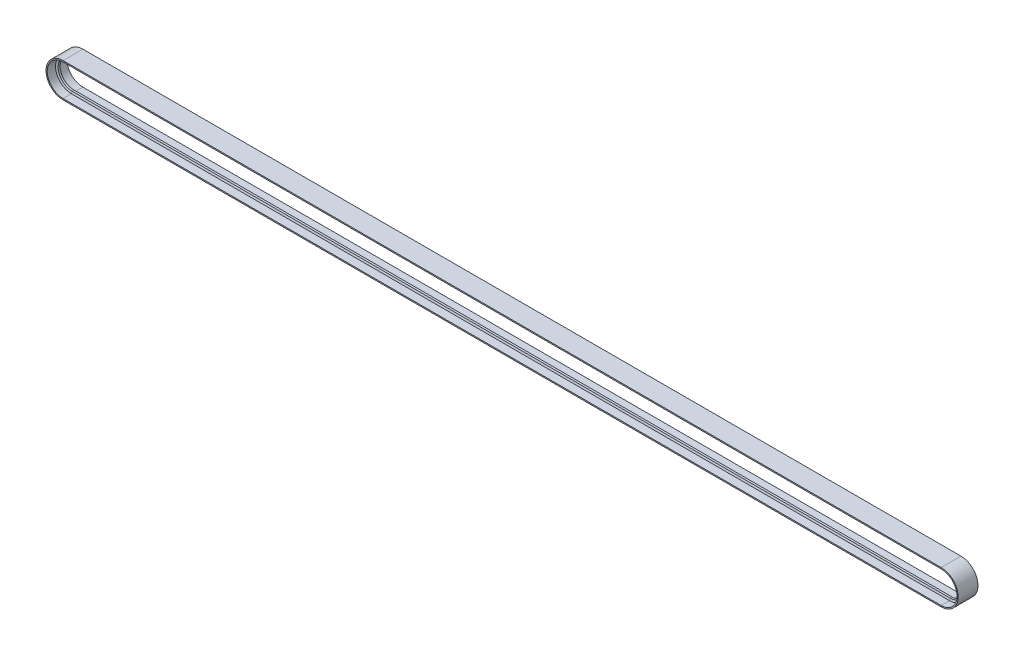
SolidWorks part; units mm, degrees
ref_plane "前视基准面" through (0, 0, 0) normal (0, 0, 1) x (1, 0, 0)
ref_plane "上视基准面" through (0, 0, 0) normal (0, 1, 0) x (1, 0, 0)
ref_plane "右视基准面" through (0, 0, 0) normal (1, 0, 0) x (0, 0, -1)
sketch "草图1" plane through (0, 0, 0) normal (0, 0, 1) x (1, 0, 0)
  line L0 (1108.5, 0) -> (-1108.5, 0) construction
  line L1 (0, 0) -> (0, 99.369) construction
  line L2 (-1108.5, 43) -> (1108.5, 43)
  line L3 (-1108.5, -43) -> (1108.5, -43)
  arc A0 (-1108.5, 43) -> (-1108.5, -43) centre (-1108.5, 0) ccw
  arc A1 (1108.5, 43) -> (1108.5, -43) centre (1108.5, 0) cw
  dimension "D1" = 86
  dimension "D2" = 2217
extrude "拉伸-薄壁1" add sketch "草图1" along normal mid plane 50 thin
sketch "草图2" plane through (0, 0, 0) normal (0, 0, 1) x (1, 0, 0)
  line L0 (-1108.5, -40) -> (1108.5, -40) construction
  line L1 (1108.5, 40) -> (-1108.5, 40) construction
  line L2 (-1108.5, -40) -> (1108.5, -40)
  line L3 (1108.5, 40) -> (-1108.5, 40)
  arc A0 (1108.5, -40) -> (1108.5, 40) centre (1108.5, 0) ccw construction
  arc A1 (-1108.5, 40) -> (-1108.5, -40) centre (-1108.5, 0) ccw construction
  arc A2 (1108.5, -40) -> (1108.5, 40) centre (1108.5, 0) ccw
  arc A3 (-1108.5, 40) -> (-1108.5, -40) centre (-1108.5, 0) ccw
sketch "草图3" plane through (0, 0, 0) normal (1, 0, 0) x (0, 0, -1)
  line L0 (0, 40) -> (0, 35) construction
  line L1 (-25, 40) -> (25, 40) construction
  line L2 (4, 40) -> (-4, 40)
  line L3 (-4, 40) -> (-2.5, 35)
  line L4 (-2.5, 35) -> (2.5, 35)
  line L5 (4, 40) -> (2.5, 35)
  dimension "D1" = 8
  dimension "D2" = 5
sweep "扫描1" add profiles "草图3" path "草图2"
